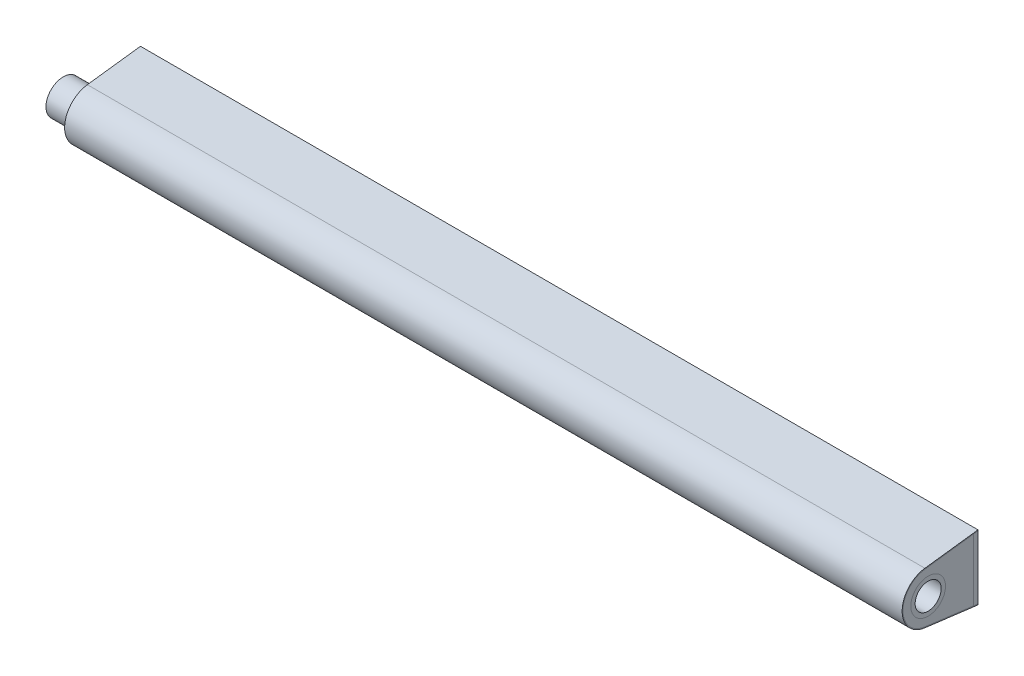
SolidWorks part; units mm, degrees
material "A3"
ref_plane "前视基准面" through (0, 0, 0) normal (0, 0, 1) x (1, 0, 0)
ref_plane "上视基准面" through (0, 0, 0) normal (0, 1, 0) x (1, 0, 0)
ref_plane "右视基准面" through (0, 0, 0) normal (1, 0, 0) x (0, 0, -1)
sketch "草图1" plane through (0, 0, 0) normal (0, 0, 1) x (1, 0, 0)
  line L1 (-966, -75) -> (966, -75)
  line L2 (-966, -75) -> (-966, 75)
  line L3 (-966, 75) -> (966, 75)
  line L4 (966, -75) -> (966, 75)
  line L5 (-966, -75) -> (966, 75) construction
  line L6 (-966, 75) -> (966, -75) construction
  point P0 (0, 0)
  dimension "D1" = 150
  dimension "D2" = 1932
extrude "凸台-拉伸1" add sketch "草图1" along normal blind 10
sketch "草图2" plane through (0, 0, 0) normal (1, 0, 0) x (0, 0, -1)
  line L0 (0, 75) -> (-122.5177, 59.5272)
  line L1 (-115, 0) -> (0, 0) construction
  line L2 (0, -75) -> (-122.5177, -59.5272)
  line L3 (0, 72.9841) -> (-122.2671, 57.5429)
  line L4 (0, -72.9841) -> (-122.2671, -57.5429)
  line L5 (0, 75) -> (0, 72.9841)
  line L6 (0, -75) -> (0, 75) construction
  line L7 (0, -75) -> (0, -72.9841)
  line L8 (0.2506, 73.0158) -> (-122.2671, 57.5429) construction
  line L9 (0.2506, -73.0158) -> (-122.2671, -57.5429) construction
  arc A0 (-122.5177, 59.5272) -> (-122.5177, -59.5272) centre (-115, 0) ccw
  arc A1 (-122.2671, 57.5429) -> (-122.2671, -57.5429) centre (-115, 0) ccw
  dimension "D1" = 120
  dimension "D2" = 115
  dimension "D3" = 2
extrude "凸台-拉伸2" add sketch "草图2" along normal mid plane 1932 separate body
sketch "草图3" plane through (0, 0, 0) normal (1, 0, 0) x (0, 0, -1)
  line L0 (0, -72.9841) -> (-122.2671, -57.5429) construction
  line L1 (-122.2671, 57.5429) -> (0, 72.9841) construction
  line L2 (0, -72.9841) -> (-122.2671, -57.5429)
  line L3 (-122.2671, 57.5429) -> (0, 72.9841)
  line L4 (0, 72.9841) -> (0, 76.6361)
  line L5 (0, 76.6361) -> (-197.0716, 76.6361)
  line L6 (-197.0716, 76.6361) -> (-197.0716, -75)
  line L7 (-197.0716, -75) -> (0, -75)
  line L8 (0, -75) -> (0, -72.9841)
  arc A0 (-122.2671, 57.5429) -> (-122.2671, -57.5429) centre (-115, 0) ccw construction
  arc A1 (-122.2671, 57.5429) -> (-122.2671, -57.5429) centre (-115, 0) ccw
extrude "切除-拉伸1" cut sketch "草图3" against normal through all both and the other way through all
sketch "草图4" plane through (966, 0, 0) normal (1, 0, 0) x (0, 0, -1)
  line L0 (0, -72.9841) -> (-122.2671, -57.5429) construction
  line L1 (-10, -71.7212) -> (-10, 71.7212) construction
  line L2 (-122.2671, 57.5429) -> (0, 72.9841) construction
  line L3 (-10, -71.7212) -> (-122.2671, -57.5429)
  line L4 (-10, -71.7212) -> (-10, 71.7212)
  line L5 (-122.2671, 57.5429) -> (-10, 71.7212)
  arc A0 (-122.2671, 57.5429) -> (-122.2671, -57.5429) centre (-115, 0) ccw construction
  arc A1 (-122.2671, 57.5429) -> (-122.2671, -57.5429) centre (-115, 0) ccw
  circle A2 centre (-115, 0) radius 40
  dimension "D1" = 80
extrude "凸台-拉伸3" add sketch "草图4" against normal blind 10 separate body
pattern_linear "阵列(线性)1" count 2 spacing 325 along (-1, 0, 0) of bodies 109
pattern_linear "阵列(线性)2" count 3 spacing 200 along (-1, 0, 0) of bodies 110
pattern_linear "阵列(线性)3" count 2 spacing 245 along (-1, 0, 0) of bodies 112
mirror "镜向1" about plane through (0, 0, 0) normal (1, 0, 0) of bodies 109 112 111 110
sketch "草图5" plane through (966, 0, 0) normal (1, 0, 0) x (0, 0, -1)
  circle A0 centre (-115, 0) radius 40 construction
  circle A1 centre (-115, 0) radius 40
  circle A2 centre (-115, 0) radius 30
  dimension "D1" = 10
extrude "凸台-拉伸4" add sketch "草图5" against normal blind 1995 separate body
ref_plane "基准面1" through (0, 0, 155) normal (0, 0, 1) x (1, 0, 0)
sketch "草图6" plane through (0, 0, 155) normal (0, 0, 1) x (1, 0, 0)
  line L0 (-1029, 40) -> (-1029, -40) construction
  line L1 (966, -57.5429) -> (966, 57.5429) construction
  circle A0 centre (801, 0) radius 5
  circle A1 centre (-869, 0) radius 5
  dimension "D1" = 10
  dimension "D2" = 160
  dimension "D3" = 165
extrude "切除-拉伸5" cut sketch "草图6" against normal mid plane 30
sketch "草图7" plane through (0, 0, 0) normal (1, 0, 0) x (0, 0, -1)
  line L0 (-10, -71.7212) -> (-10, 71.7212) construction
  line L1 (-10, 5) -> (-75, 5)
  line L2 (-10, 5) -> (-10, -5)
  line L3 (-10, -5) -> (-75, -5)
  line L4 (-75, 5) -> (-75, -5)
  circle A0 centre (-115, 0) radius 40 construction
  point P6 (-10, 0)
  dimension "D1" = 10
extrude "凸台-拉伸5" add sketch "草图7" along normal mid plane 1912 separate body
